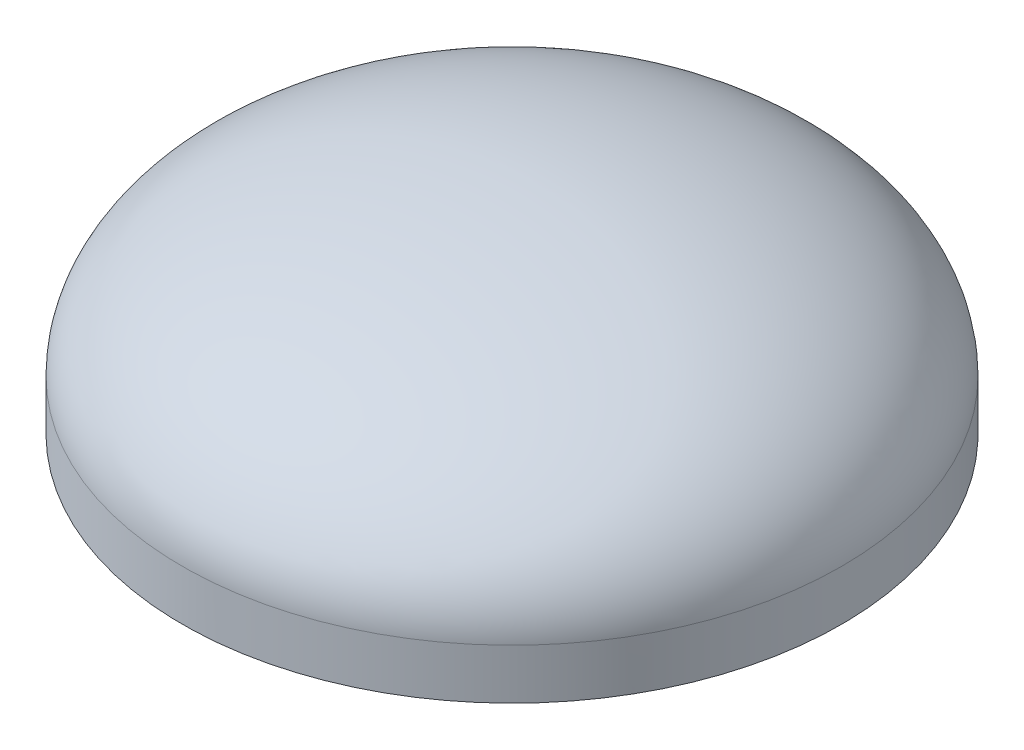
from build123d import *


with BuildPart() as part:
    # Sketch3 → Revolve2 (revolve)
    with BuildSketch(Plane.XY, mode=Mode.PRIVATE) as revolve2_sk:
        with BuildLine():
            Line((-162.5, 0), (-162.5, -24.75))
            Line((-162.5, -24.75), (-159.5, -24.75))
            Line((-159.5, -24.75), (-159.5, 0))
            add(Edge.make_bspline(
                [(0, 78.25), (-159.5, 78.25), (-159.5, 0)],
                knots=[1.570796327, 1.570796327, 1.570796327, 3.141592654, 3.141592654, 3.141592654], degree=2, weights=[1, 0.707106781, 1]))
            Line((0, 78.25), (0, 81.25))
            add(Edge.make_bspline(
                [(0, 81.25), (-162.5, 81.25), (-162.5, 0)],
                knots=[1.570796327, 1.570796327, 1.570796327, 3.141592654, 3.141592654, 3.141592654], degree=2, weights=[1, 0.707106781, 1]))
        make_face()
    revolve(revolve2_sk.sketch.rotate(Axis((0, 0, 0), (0, 1, 0)), 270), axis=Axis((0, 0, 0), (0, 1, 0)))


solid = part.part
